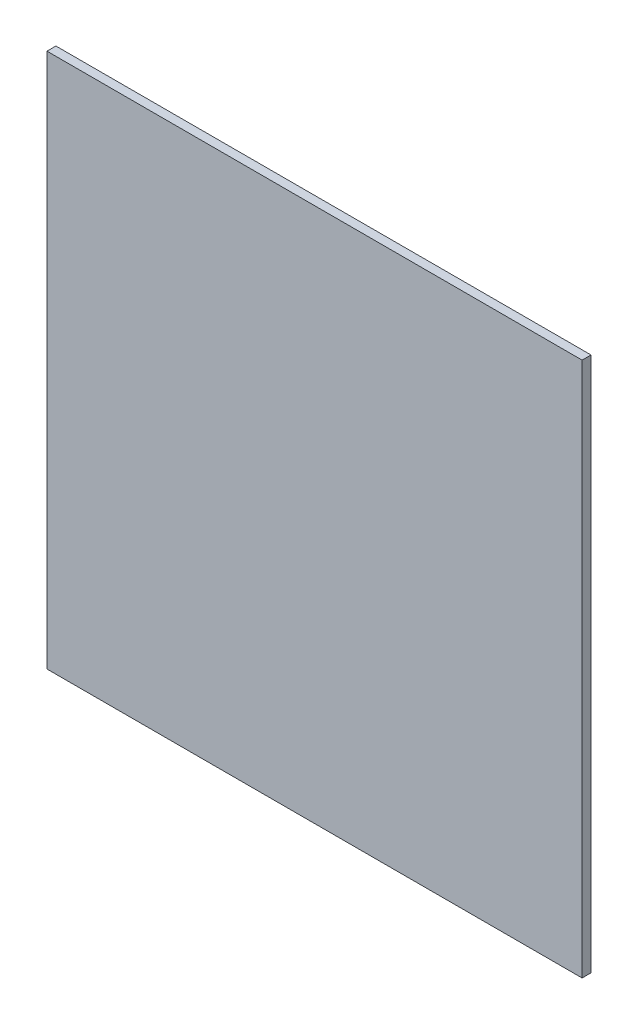
from build123d import *

# Parameters (mm, degrees)
SKETCH1_W           = 600
SKETCH1_H           = 600
BOSS_EXTRUDE1_DEPTH = 10


with BuildPart() as part:
    # Sketch1 → Boss-Extrude1 (new body)
    with BuildSketch(Plane.XY):
        with Locations((300, 300)):
            Rectangle(SKETCH1_W, SKETCH1_H)
    extrude(amount=BOSS_EXTRUDE1_DEPTH)


solid = part.part
